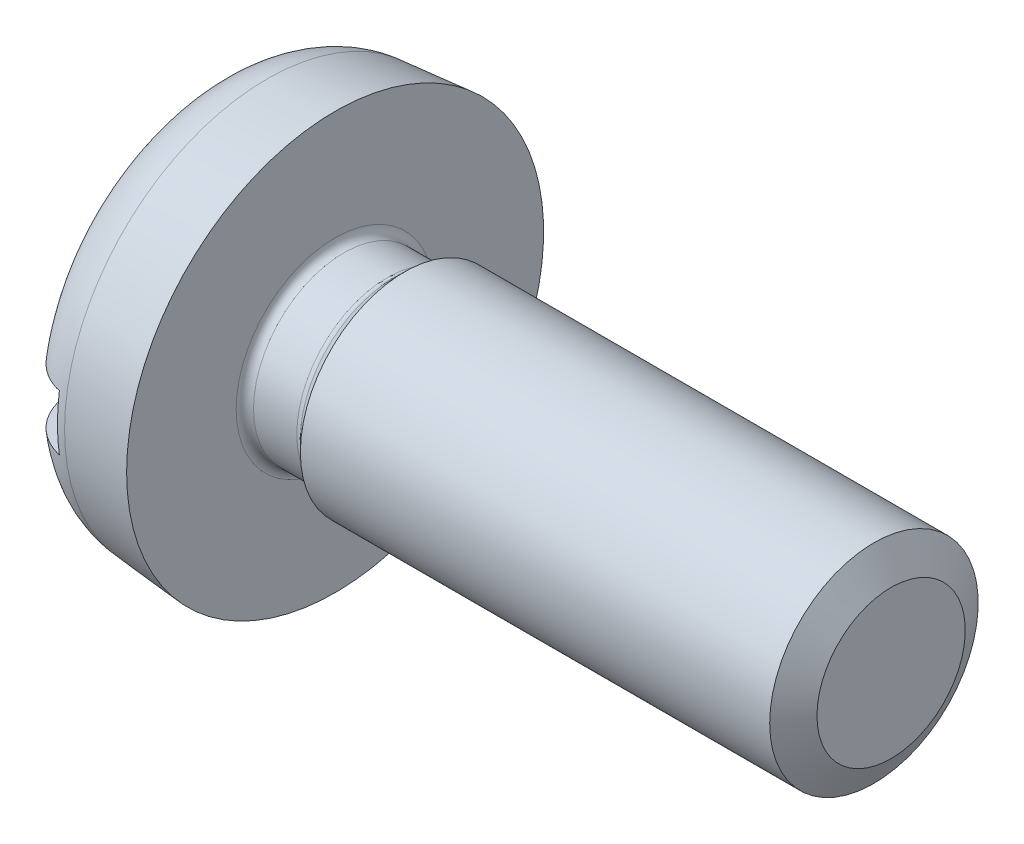
SolidWorks part; units mm, degrees
ref_plane "Front Plane" through (0, 0, 0) normal (0, 0, 1) x (1, 0, 0)
ref_plane "Top Plane" through (0, 0, 0) normal (0, 1, 0) x (1, 0, 0)
ref_plane "Right Plane" through (0, 0, 0) normal (1, 0, 0) x (0, 0, -1)
sketch "Dimensioned Sketch" plane through (0, 0, 0) normal (0, 0, 1) x (1, 0, 0)
  line L0 (0, 0) -> (16, 0) construction
  line L1 (16, 0) -> (16, 6) construction
  line L2 (0, 0) -> (0, 12) construction
  point P5 (15, 0)
  point P6 (2, 0)
  point P7 (3.6, 0)
  point P8 (0, 6.8)
  point P9 (5.2, 0)
  point P12 (0, 11.75)
  point P13 (7, 0)
  point P14 (8.4, 0)
  point P15 (9.8, 0)
  dimension "dk" = 12
  dimension "d" = 6
  dimension "l" = 16
  dimension "P" = 1
  dimension "a" = 2
  dimension "k" = 3.6
  dimension "r" = 0.25
  dimension "da" = 6.8
  dimension "n" = 1.6
  dimension "r1" = 1.8
  dimension "t" = 1.4
  dimension "w" = 1.4
sketch "Sketch2" plane through (0, 0, 0) normal (0, 0, 1) x (1, 0, 0)
  line L0 (-3.442, 0) -> (0, 0) construction
  line L1 (0, 0) -> (19.6, 0)
  line L2 (19.6, 0) -> (19.6, 3)
  line L3 (19.6, 3) -> (5.6, 3)
  line L4 (5.6, 3) -> (5.198, 2.598)
  line L5 (3.6, 6) -> (3.6, 2.598)
  line L6 (3.6, 6) -> (-0.815, 6) construction
  line L7 (3.6, 6) -> (0, 5.685)
  line L8 (3.6, 2.598) -> (5.198, 2.598)
  line L9 (0, 5.685) -> (0, 0)
  dimension "D1" = 5.196
  dimension "d" = 6
  dimension "D2" = 12
  dimension "a" = 2
  dimension "D3" = 45
  dimension "D4" = 16
  dimension "D5" = 5
  dimension "D6" = 3.6
revolve "Base-Revolve" add sketch "Sketch2" angle 360 about L0
cosmetic thread "Cosmetic Thread1" parameters "D2"=5.196
fillet "Fillet1" radius 0.25 2 edges at (3.6, 0, 2.598) (5.198, 0, 2.598)
fillet "Fillet2" radius 1.8 1 edges at (0, 0, 5.685)
sketch "Sketch5" plane through (0, 0, 0) normal (1, 0, 0) x (0, 0, -1)
  line L0 (0, 0) -> (-6, 0) construction
  line L1 (6, 0.8) -> (-6, 0.8)
  line L2 (6, -0.8) -> (-6, -0.8)
  line L3 (-6, 0.8) -> (-6, -0.8)
  line L4 (6, 0.8) -> (6, -0.8)
  line L5 (0, 0) -> (0, 6) construction
  circle A0 centre (0, 0) radius 6 construction
  point P2 (0, 0.8)
  point P12 (0, -0.8)
  dimension "D1" = 1.6
extrude "Cut-Extrude1" cut sketch "Sketch5" along normal blind 1.4
sketch "Sketch3" plane through (0, 0, 0) normal (0, 0, 1) x (1, 0, 0)
  line L0 (19.1054, 3) -> (20.1054, 3)
  line L1 (20.1054, 3) -> (19.6, 2.134)
  line L2 (19.6, 2.134) -> (19.1054, 3)
  line L3 (19.6, 3) -> (5.6, 3) construction
  line L4 (19.6, -3) -> (19.6, 3) construction
  line L5 (-0.1226, 0) -> (5.6936, 0) construction
  line L6 (-3.442, 0) -> (0, 0) construction
  dimension "D1" = 60
  dimension "P" = 1
  dimension "D3" = 0.866
revolve "Cut-Revolve1" cut sketch "Sketch3" angle 360 about L5
pattern_linear "LPattern1" [suppressed] count 15 spacing 1 along (1, 0, 0)
